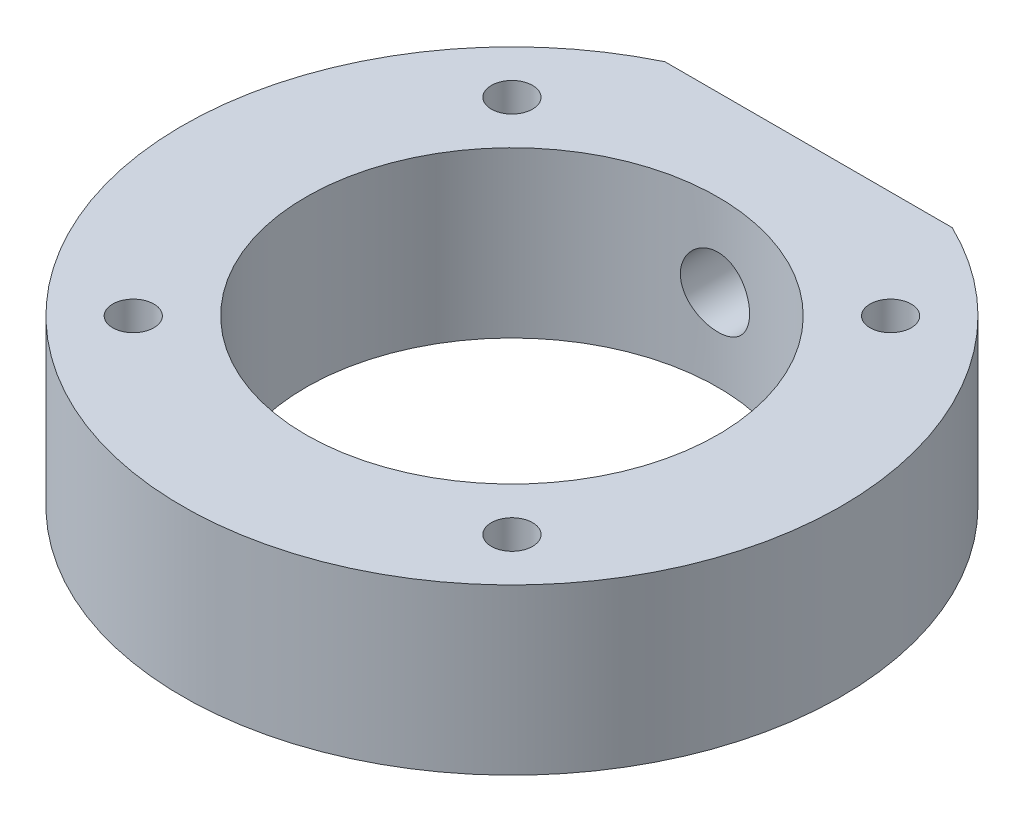
SolidWorks part; units mm, degrees
ref_plane "Front Plane" through (0, 0, 0) normal (0, 0, 1) x (1, 0, 0)
ref_plane "Top Plane" through (0, 0, 0) normal (0, 1, 0) x (1, 0, 0)
ref_plane "Right Plane" through (0, 0, 0) normal (1, 0, 0) x (0, 0, -1)
sketch "Sketch1" plane through (0, 0, 0) normal (0, 1, 0) x (1, 0, 0)
  circle A0 centre (0, 0) radius 12.5
  circle A1 centre (0, 0) radius 20
  dimension "D1" = 25
  dimension "D2" = 40
extrude "Boss-Extrude1" add sketch "Sketch1" along normal blind 10
sketch "Sketch2" plane through (0, 10, 0) normal (0, 1, 0) x (1, 0, 0)
  line L0 (8.7178, 18) -> (-8.7178, 18)
  circle A0 centre (0, 0) radius 20 construction
  arc A1 (8.7178, 18) -> (-8.7178, 18) centre (0, 0) ccw
  dimension "D1" = 18
extrude "Cut-Extrude1" cut sketch "Sketch2" against normal through all
hole_wizard "M5 Tapped Hole1" positions "Sketch3" profile "Sketch4" tap size "M5" standard "GB"
sketch "Sketch3" plane through (0, 0, -18) normal (0, 0, -1) x (-1, 0, 0)
  line L0 (8.7178, 0) -> (8.7178, 10) construction
  point P0 (0, 5)
  point P6 (8.7178, 5)
sketch "Sketch4" plane through (0, 5, -18) normal (1, 0, 0) x (0, 1, 0)
  line L0 (0, 0) -> (0, 5.5)
  line L1 (0, 5.5) -> (2.1, 5.5)
  line L2 (2.1, 5.5) -> (2.1, 0)
  line L5 (2.1, 0) -> (0, 0)
  line L11 (0, -6.35) -> (0, 107.95) construction
  dimension "通孔螺纹孔钻头直径" = 4.2
  dimension "通孔螺纹孔钻头深度" = 5.5
cosmetic thread "Cosmetic Thread1" parameters "D2"=5
hole_wizard "M3 Tapped Hole1" positions "Sketch5" profile "Sketch6" tap size "M3" standard "GB" end condition up to next
sketch "Sketch5" plane through (0, 0, 0) normal (0, -1, 0) x (-1, 0, 0)
  line L0 (0, 0) -> (50000, 0) construction
  line L1 (0, 0) -> (0, -50000) construction
  line L4 (-14.1421, 14.1421) -> (-8.8388, 8.8388) construction
  arc A0 (-8.7178, 18) -> (8.7178, 18) centre (0, 0) ccw construction
  circle A1 centre (0, 0) radius 12.5 construction
  point P0 (-11.4905, 11.4905)
  point P27 (-11.4905, 11.4905)
  point P28 (11.4905, 11.4905)
  point P29 (-11.4905, -11.4905)
  point P30 (11.4905, -11.4905)
  dimension "D1" = 45
  dimension "D2" = 7.5
sketch "Sketch6" plane through (11.4905, 0, -11.4905) normal (1, 0, 0) x (0, 0, -1)
  line L0 (0, 0) -> (0, 10)
  line L1 (0, 10) -> (1.25, 10)
  line L2 (1.25, 10) -> (1.25, 0)
  line L5 (1.25, 0) -> (0, 0)
  line L11 (0, -6.35) -> (0, 107.95) construction
  dimension "通孔螺纹孔钻头直径" = 2.5
  dimension "通孔螺纹孔钻头深度" = 10
cosmetic thread "Cosmetic Thread2" parameters "D2"=3
cosmetic thread "Cosmetic Thread3" parameters "D2"=3
cosmetic thread "Cosmetic Thread4" parameters "D2"=3
cosmetic thread "Cosmetic Thread5" parameters "D2"=3
